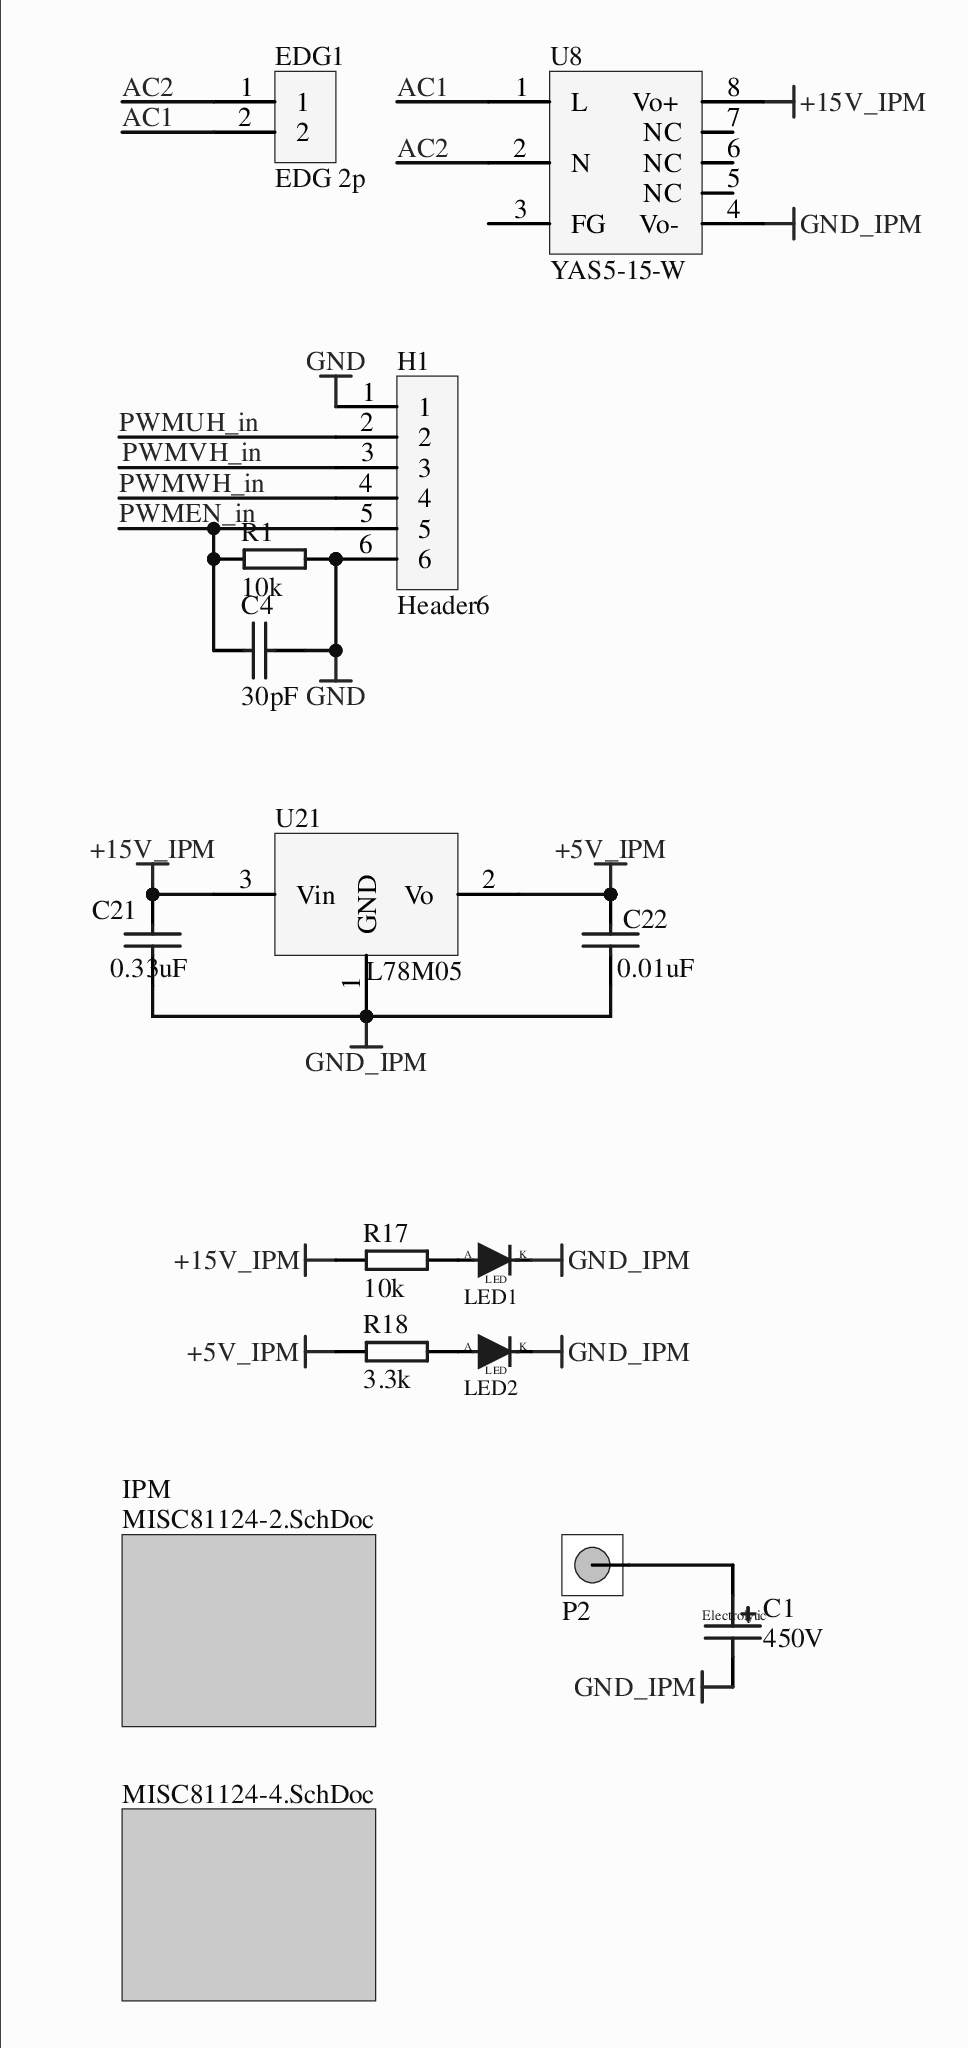
[diagram p0: MISC81124-5.SchDoc]
# Altium project MISC81124-3.PrjPcb
3 sheets, 58 parts. Net scope: global (net labels, ports and power ports of the same name join across sheets).
Board file: MISC81124.PcbDoc
Sheets:
  MISC81124-5.SchDoc
    IPM = MISC81124-2.SchDoc
     = MISC81124-4.SchDoc

## Sheet MISC81124-5.SchDoc
size A4

### Parts
C1  450V  [ElecCap_450V]
C4  30pF  [0805]
C21  0.33uF  [0805]
C22  0.01uF  [0805]
EDG1  EDG 2p  [EDGCon_2p_3.81mm]
H1  Header6  [EDGCon_6P_5.08mm]
LED1  LED  [0805_LED]  (value not drawn)
LED2  LED  [0805_LED]  (value not drawn)
P2  PCBTerminator  [PCBTerminator]  (value not drawn)
R1  10k  [0805]
R17  10k  [0805]
R18  3.3k  [0805]
U8  YAS5-15-W  [YAS5]
U21  L78M05  [TO-252-2(DPAK)]

### Sub-sheets
IPM = MISC81124-2.SchDoc: no entries
? = MISC81124-4.SchDoc: no entries

### Nets
+5V_IPM: C22.2 R18.2 U21.2(Vo)
+15V_IPM: C21.2 R17.2 U8.8(Vo+) U21.3(Vin)
GND: C4.1 H1.1 H1.6 R1.1
GND_IPM: C1.2 C21.1 C22.1 LED1.K LED2.K U8.4(Vo-) U21.1(GND)  [project net IPM_N]
AC1: EDG1.2 U8.1(L)
AC2: EDG1.1 U8.2(N)
PWMEN_in: C4.2 H1.5 R1.2
PWMUH_in: H1.2
PWMVH_in: H1.3
PWMWH_in: H1.4
NetC1_1: C1.1 P2.1
NetLED1_A: LED1.A R17.1
NetLED2_A: LED2.A R18.1

Not connected (* = marked no-connect by the designer): U8 3(FG) 5(NC) 6(NC) 7(NC)

### Library data of the parts
C1 = ELECTROCap: Electrolytic Capacitor(Pin1 Positive)
C4 C21 C22 = CAP: Capacitor
P2 = PCBTerminator: PCB terminal for high current
R1 R17 R18 = RES2
U8 = YAS5
U21 = LM1085ISX-3.3

## Sheet MISC81124-2.SchDoc
size 127 x 139 mm
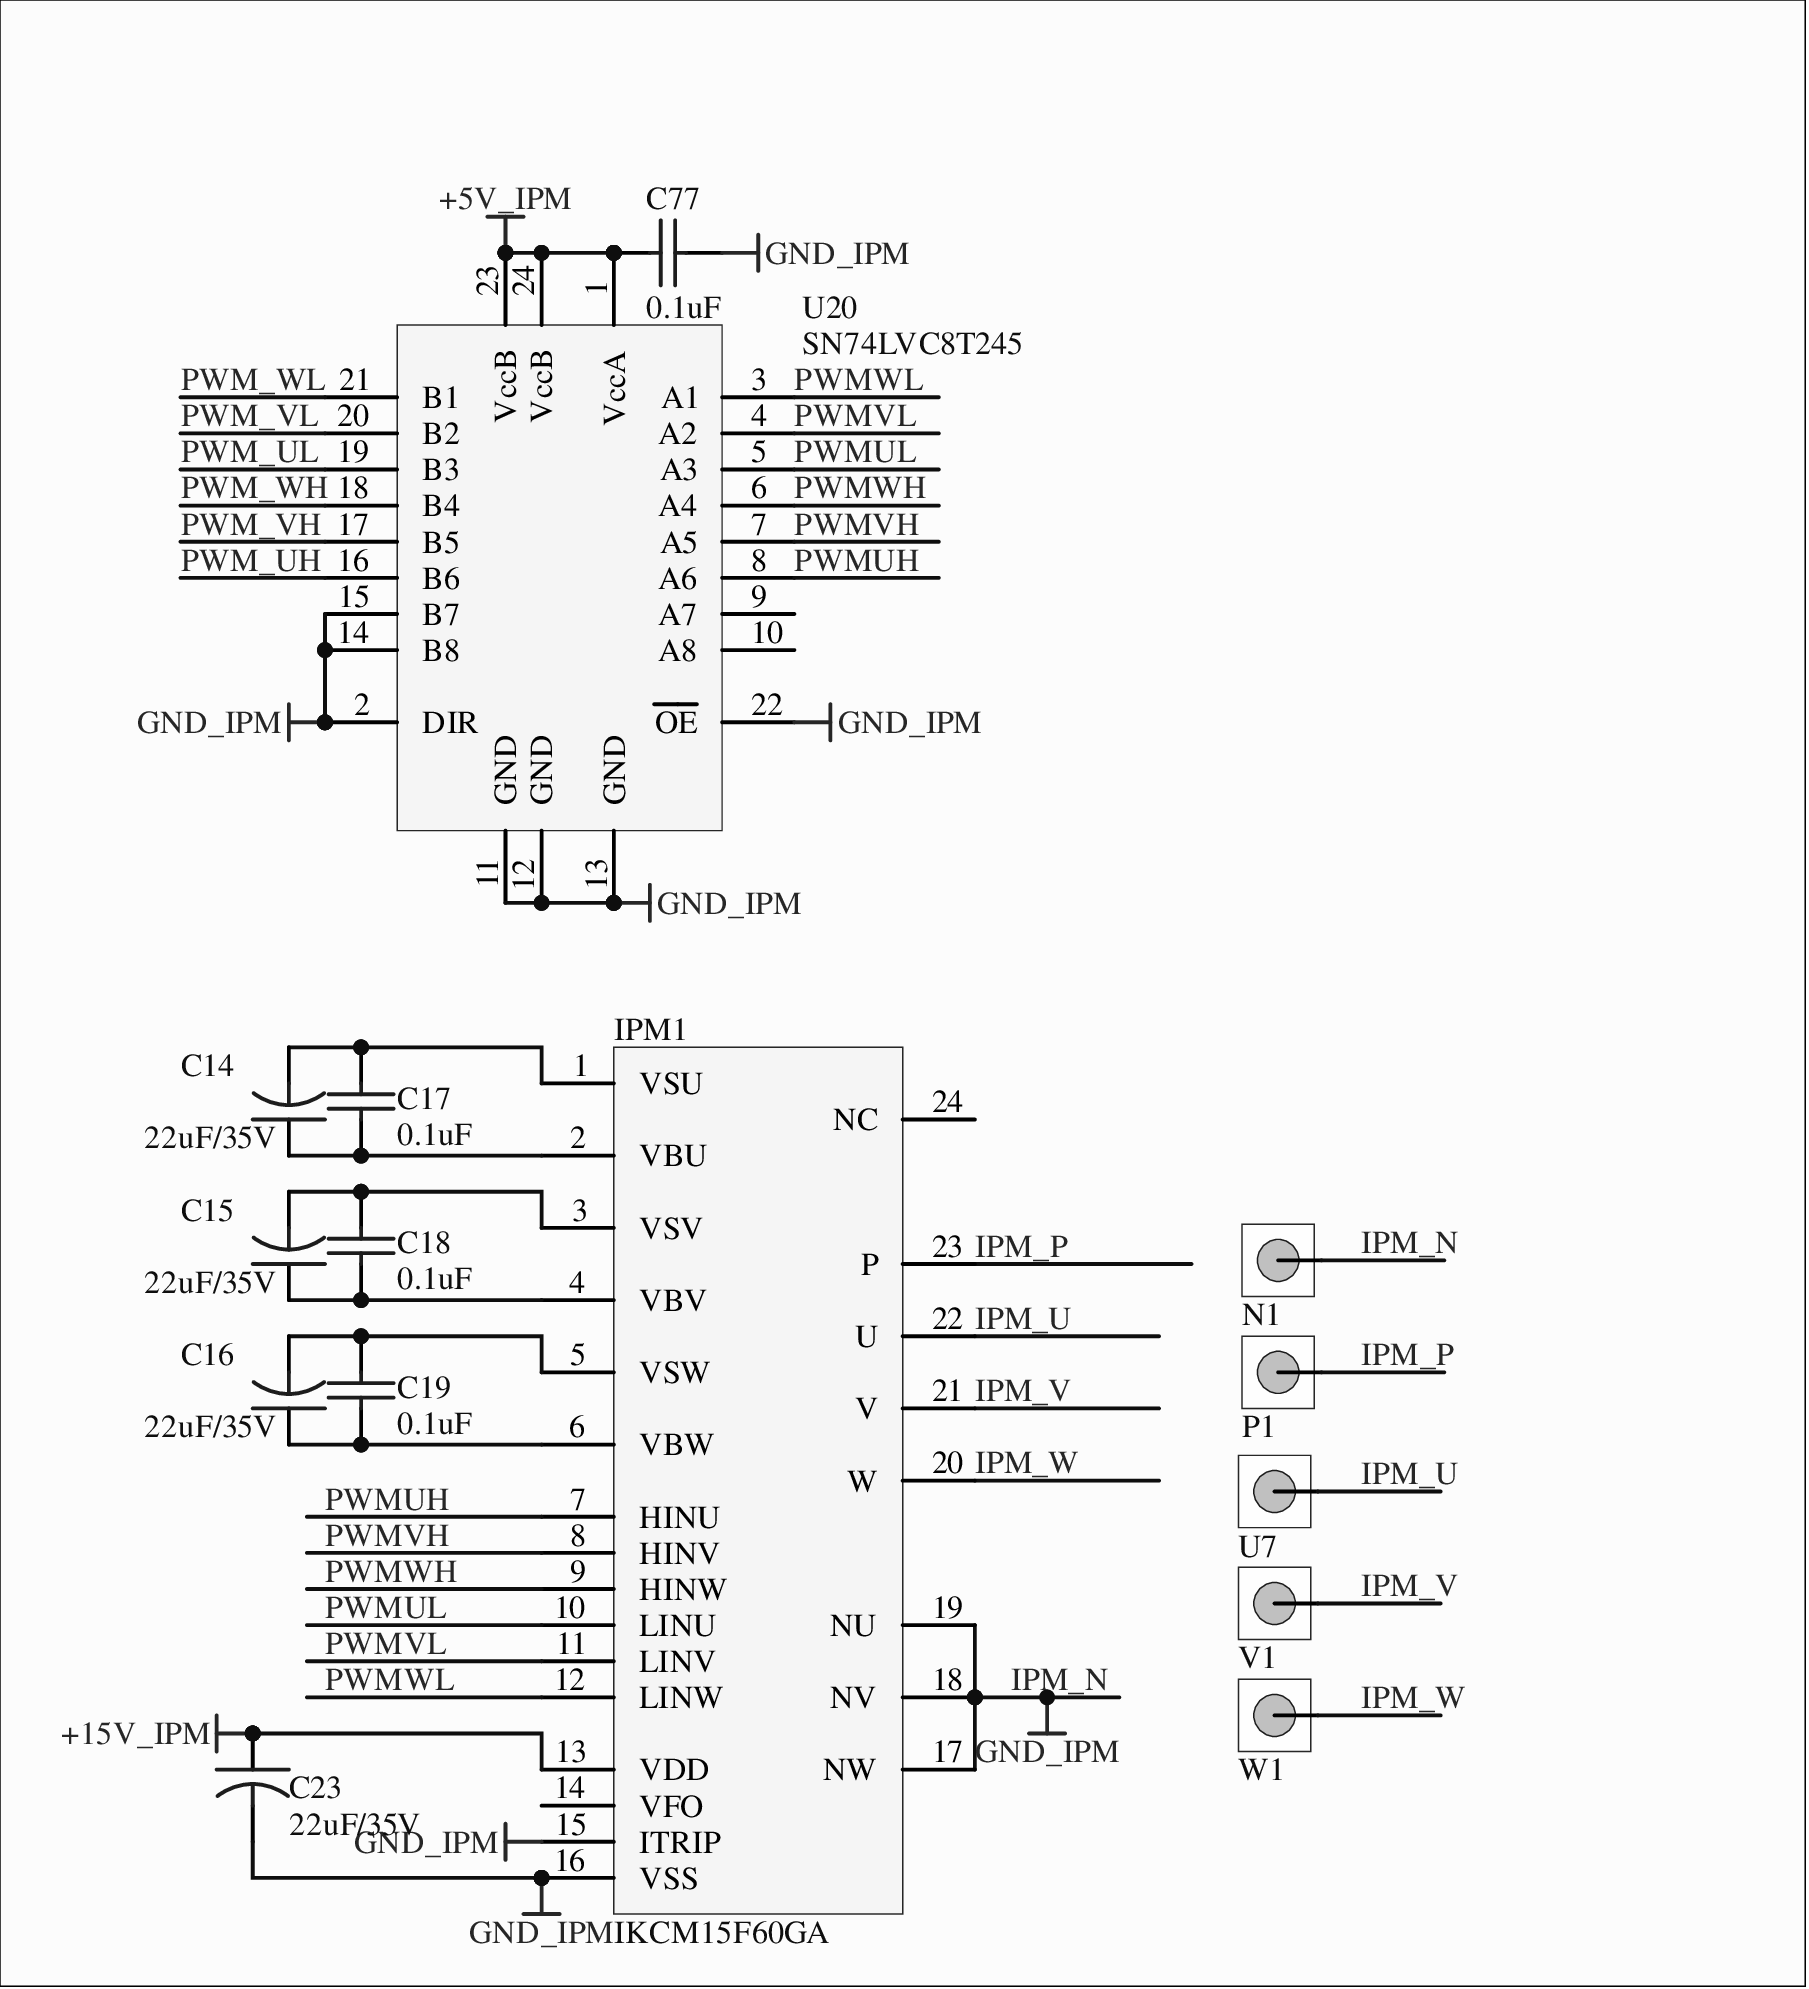
[diagram p1: MISC81124-2.SchDoc]

### Parts
C14  22uF/35V  [7343_CASE-D]
C15  22uF/35V  [7343_CASE-D]
C16  22uF/35V  [7343_CASE-D]
C17  0.1uF  [0805]
C18  0.1uF  [0805]
C19  0.1uF  [0805]
C23  22uF/35V  [7343_CASE-D]
C77  0.1uF  [0805]
IPM1  IKCM15F60GA  [IKCM15F60GA]
N1  PCBTerminator  [PCBTerminator]  (value not drawn)
P1  PCBTerminator  [PCBTerminator]  (value not drawn)
U7  PCBTerminator  [PCBTerminator]  (value not drawn)
U20  SN74LVC8T245  [SN74LVC8T245_TSSOP24]
V1  PCBTerminator  [PCBTerminator]  (value not drawn)
W1  PCBTerminator  [PCBTerminator]  (value not drawn)

### Nets
+5V_IPM: C77.1 U20.1(VccA) U20.23(VccB) U20.24(VccB)
+15V_IPM: C23.1 IPM1.13(VDD)
IPM_N: C23.2 C77.2 IPM1.15(ITRIP) IPM1.16(VSS) IPM1.17(NW) IPM1.18(NV) IPM1.19(NU) N1.1 U20.2(DIR) U20.11(GND) U20.12(GND) U20.13(GND) U20.14(B8) U20.15(B7) U20.22(~{OE})  [also labelled GND_IPM]
IPM_P: IPM1.23(P) P1.1
IPM_U: IPM1.22(U) U7.1
IPM_V: IPM1.21(V) V1.1
IPM_W: IPM1.20(W) W1.1
PWM_UH: U20.16(B6)
PWM_UL: U20.19(B3)
PWM_VH: U20.17(B5)
PWM_VL: U20.20(B2)
PWM_WH: U20.18(B4)
PWM_WL: U20.21(B1)
PWMUH: IPM1.7(HINU) U20.8(A6)
PWMUL: IPM1.10(LINU) U20.5(A3)
PWMVH: IPM1.8(HINV) U20.7(A5)
PWMVL: IPM1.11(LINV) U20.4(A2)
PWMWH: IPM1.9(HINW) U20.6(A4)
PWMWL: IPM1.12(LINW) U20.3(A1)
NetC14_1: C14.1 C17.1 IPM1.2(VBU)
NetC14_2: C14.2 C17.2 IPM1.1(VSU)
NetC15_1: C15.1 C18.1 IPM1.4(VBV)
NetC15_2: C15.2 C18.2 IPM1.3(VSV)
NetC16_1: C16.1 C19.1 IPM1.6(VBW)
NetC16_2: C16.2 C19.2 IPM1.5(VSW)

Not connected (* = marked no-connect by the designer): IPM1 14(VFO)* 24(NC); U20 9(A7) 10(A8)

### Library data of the parts
C14-C16 C23 = TaCap_D
C17-C19 C77 = CAP: Capacitor
N1 P1 U7 V1 W1 = PCBTerminator: PCB terminal for high current
U20 = SN74LVC8T245: TI SN74LVC8T245PWR

## Sheet MISC81124-4.SchDoc
size A4 portrait
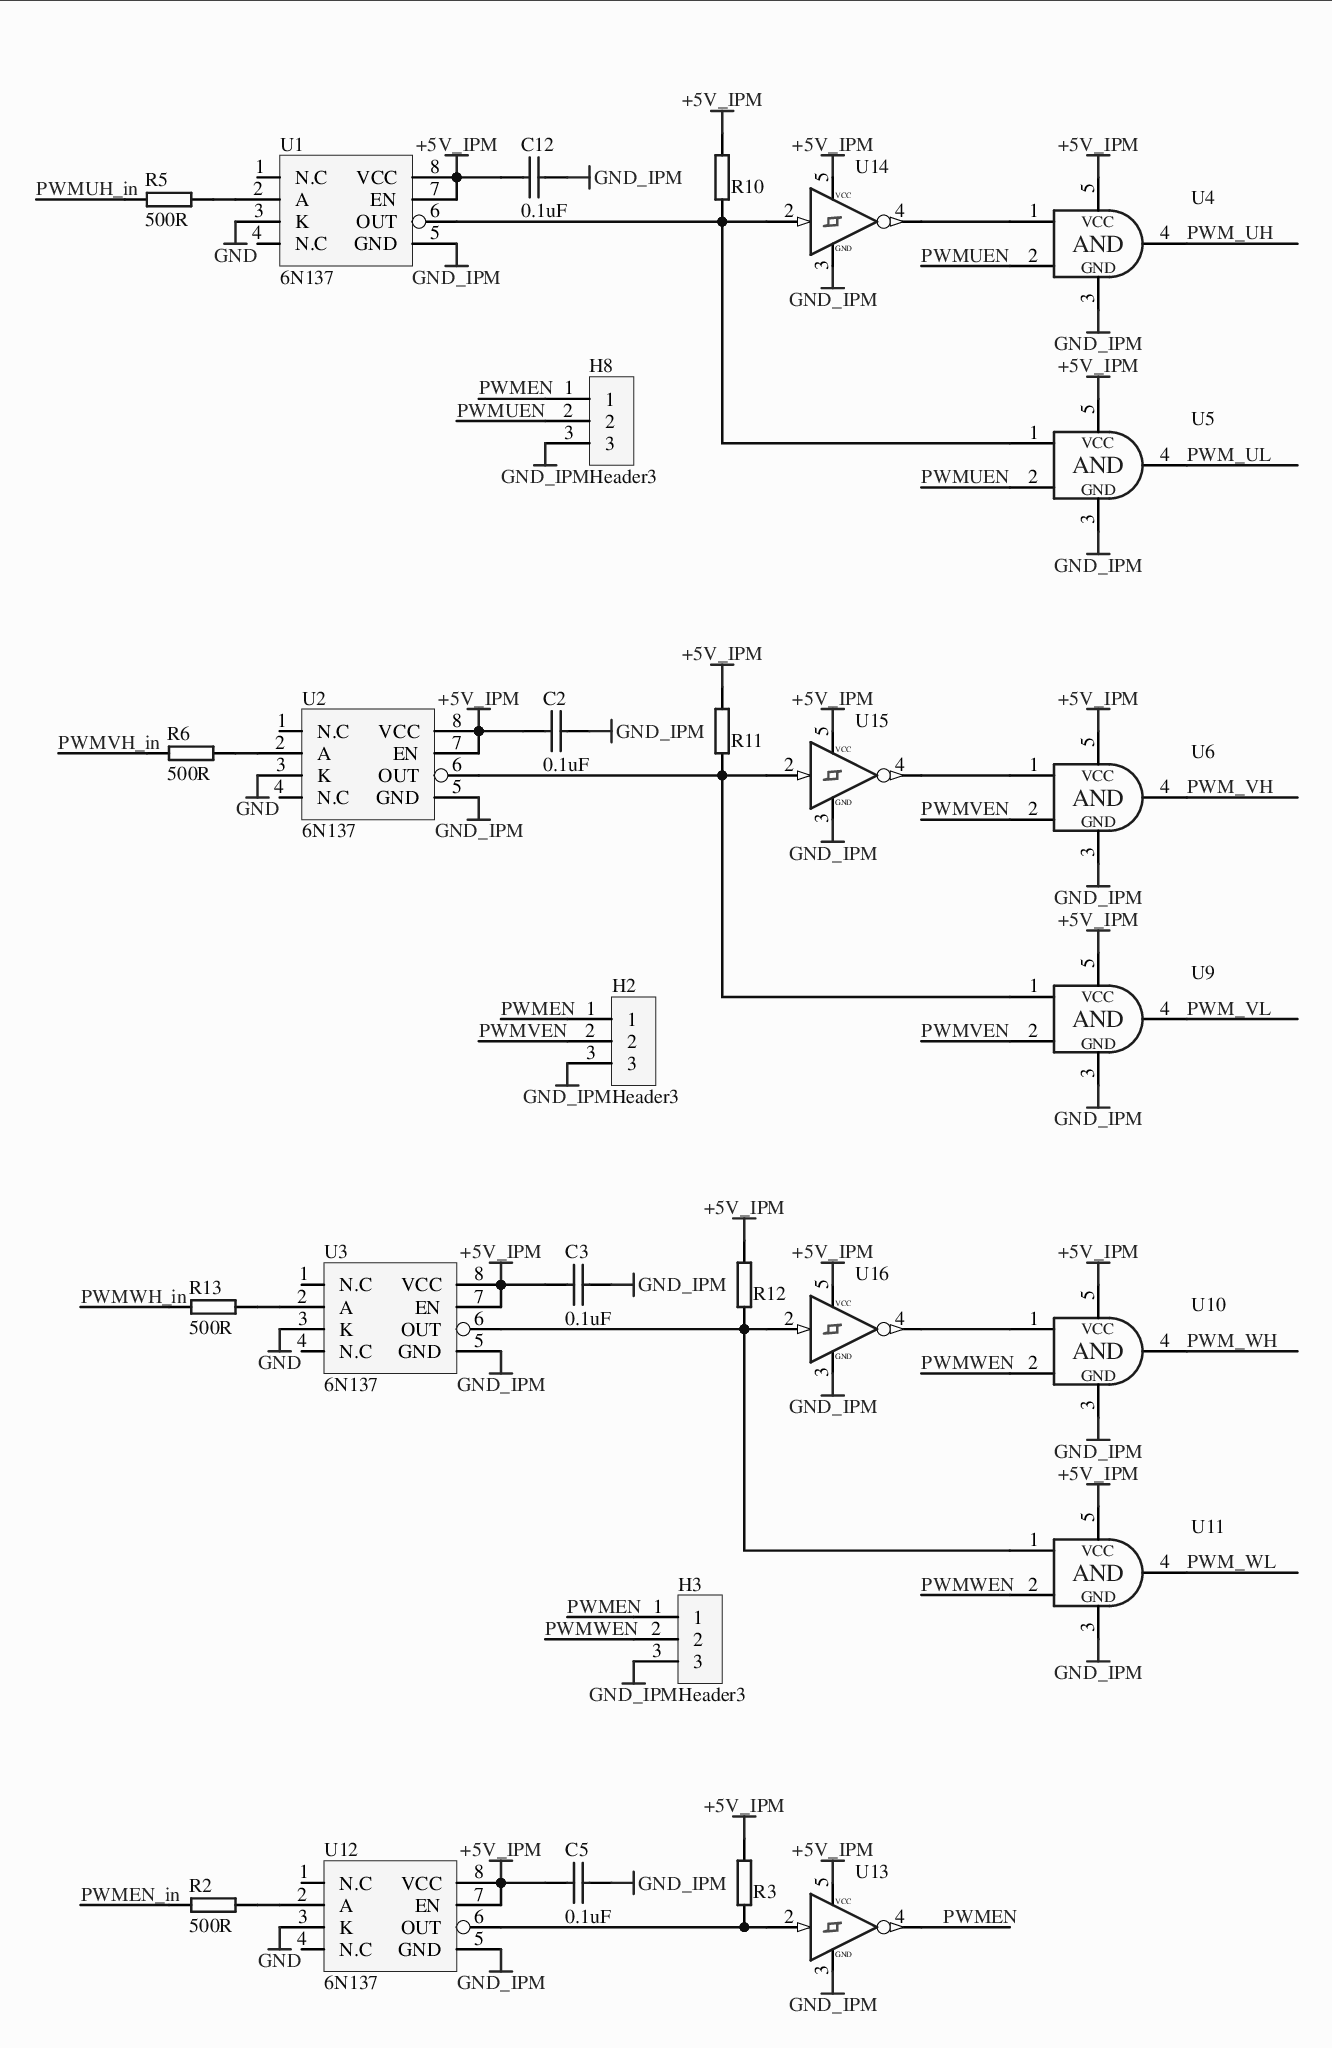
[diagram p2: MISC81124-4.SchDoc]

### Parts
C2  0.1uF  [0805]
C3  0.1uF  [0805]
C5  0.1uF  [0805]
C12  0.1uF  [0805]
H2  Header3  [PinHeader3_2.54mm]
H3  Header3  [PinHeader3_2.54mm]
H8  Header3  [PinHeader3_2.54mm]
R2  500R  [1206]
R3  10k  [0805]  (value not drawn)
R5  500R  [1206]
R6  500R  [1206]
R10  10k  [0805]  (value not drawn)
R11  10k  [0805]  (value not drawn)
R12  10k  [0805]  (value not drawn)
R13  500R  [1206]
U1  6N137  [DIP-8]
U2  6N137  [DIP-8]
U3  6N137  [DIP-8]
U4  SN74AHC1G08  [SOT-23-5]  (value not drawn)
U5  SN74AHC1G08  [SOT-23-5]  (value not drawn)
U6  SN74AHC1G08  [SOT-23-5]  (value not drawn)
U9  SN74AHC1G08  [SOT-23-5]  (value not drawn)
U10  SN74AHC1G08  [SOT-23-5]  (value not drawn)
U11  SN74AHC1G08  [SOT-23-5]  (value not drawn)
U12  6N137  [DIP-8]
U13  SN74AHC1G04  [SOT-23-5]  (value not drawn)
U14  SN74AHC1G04  [SOT-23-5]  (value not drawn)
U15  SN74AHC1G04  [SOT-23-5]  (value not drawn)
U16  SN74AHC1G04  [SOT-23-5]  (value not drawn)

### Nets
+5V_IPM: C2.2 C3.2 C5.2 C12.2 R3.2 R10.2 R11.2 R12.2 U1.7(EN) U1.8(VCC) U2.7(EN) U2.8(VCC) U3.7(EN) U3.8(VCC) U4.5(VCC) U5.5(VCC) U6.5(VCC) U9.5(VCC) U10.5(VCC) U11.5(VCC) U12.7(EN) U12.8(VCC) U13.5(VCC) U14.5(VCC) U15.5(VCC) U16.5(VCC)
GND: U1.3(K) U2.3(K) U3.3(K) U12.3(K)
GND_IPM: C2.1 C3.1 C5.1 C12.1 H2.3 H3.3 H8.3 U1.5(GND) U2.5(GND) U3.5(GND) U4.3(GND) U5.3(GND) U6.3(GND) U9.3(GND) U10.3(GND) U11.3(GND) U12.5(GND) U13.3(GND) U14.3(GND) U15.3(GND) U16.3(GND)  [project net IPM_N]
PWM_UH: U4.4(Y)
PWM_UL: U5.4(Y)
PWM_VH: U6.4(Y)
PWM_VL: U9.4(Y)
PWM_WH: U10.4(Y)
PWM_WL: U11.4(Y)
PWMEN: H2.1 H3.1 H8.1 U13.4(Y)
PWMEN_in: R2.2
PWMUEN: H8.2 U4.2(B) U5.2(B)
PWMUH_in: R5.2
PWMVEN: H2.2 U6.2(B) U9.2(B)
PWMVH_in: R6.2
PWMWEN: H3.2 U10.2(B) U11.2(B)
PWMWH_in: R13.2
NetR2_1: R2.1 U12.2(A)
NetR3_1: R3.1 U12.6(OUT) U13.2(A)
NetR5_1: R5.1 U1.2(A)
NetR6_1: R6.1 U2.2(A)
NetR10_1: R10.1 U1.6(OUT) U5.1(A) U14.2(A)
NetR11_1: R11.1 U2.6(OUT) U9.1(A) U15.2(A)
NetR12_1: R12.1 U3.6(OUT) U11.1(A) U16.2(A)
NetR13_1: R13.1 U3.2(A)
NetU4_1: U4.1(A) U14.4(Y)
NetU6_1: U6.1(A) U15.4(Y)
NetU10_1: U10.1(A) U16.4(Y)

Not connected (* = marked no-connect by the designer): U1 1(N.C) 4(N.C); U2 1(N.C) 4(N.C); U3 1(N.C) 4(N.C); U12 1(N.C) 4(N.C)

### Library data of the parts
C2 C3 C5 C12 = CAP: Capacitor
R2 R3 R5 R6 R10-R13 = RES2
U1-U3 U12 = 6N137: High-speed optocoupler
U4-U6 U9-U11 = SN74AHC1G08: Single 2-Input Positive-AND Buffer
U13-U16 = SN74AHC1G04: Single Input Inverter

## Nets that join several sheets
+5V_IPM: MISC81124-5 (C22.2 R18.2 U21.2), MISC81124-2 (C77.1 U20.1 U20.23 U20.24), MISC81124-4 (26 pins)
+15V_IPM: MISC81124-5 (C21.2 R17.2 U8.8 U21.3), MISC81124-2 (C23.1 IPM1.13)
GND: MISC81124-5 (C4.1 H1.1 H1.6 R1.1), MISC81124-4 (U1.3 U2.3 U3.3 U12.3)
IPM_N: MISC81124-5 (7 pins), MISC81124-2 (15 pins), MISC81124-4 (21 pins)
PWM_UH: MISC81124-2 (U20.16), MISC81124-4 (U4.4)
PWM_UL: MISC81124-2 (U20.19), MISC81124-4 (U5.4)
PWM_VH: MISC81124-2 (U20.17), MISC81124-4 (U6.4)
PWM_VL: MISC81124-2 (U20.20), MISC81124-4 (U9.4)
PWM_WH: MISC81124-2 (U20.18), MISC81124-4 (U10.4)
PWM_WL: MISC81124-2 (U20.21), MISC81124-4 (U11.4)
PWMEN_in: MISC81124-5 (C4.2 H1.5 R1.2), MISC81124-4 (R2.2)
PWMUH_in: MISC81124-5 (H1.2), MISC81124-4 (R5.2)
PWMVH_in: MISC81124-5 (H1.3), MISC81124-4 (R6.2)
PWMWH_in: MISC81124-5 (H1.4), MISC81124-4 (R13.2)